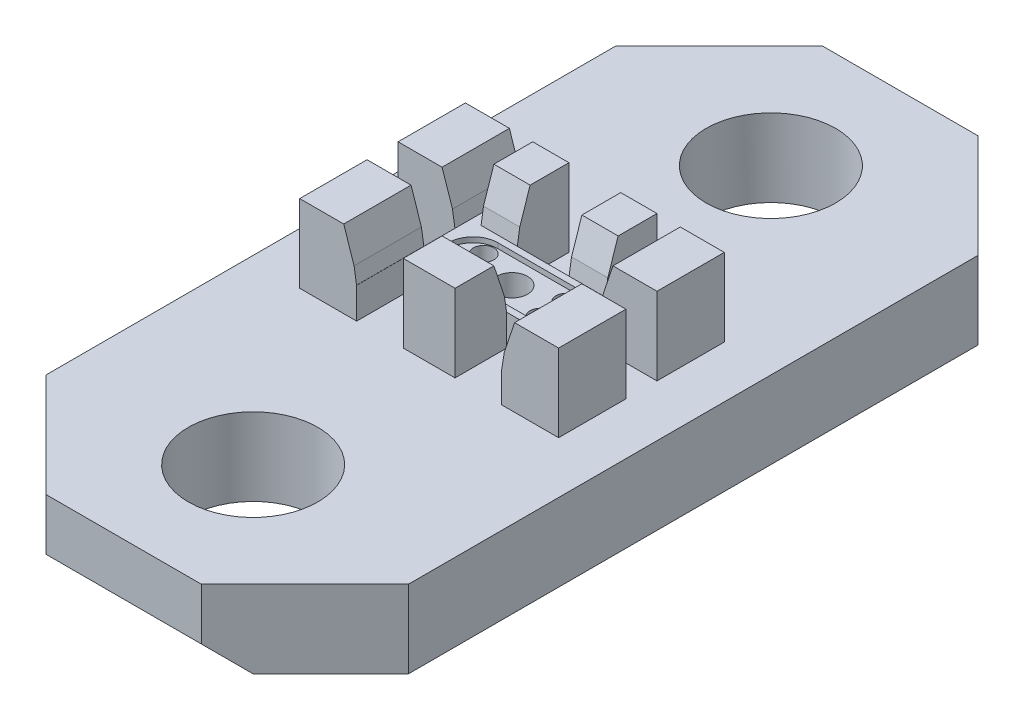
from build123d import *
from OCP.BRepFilletAPI import BRepFilletAPI_MakeChamfer

# Parameters (mm, degrees)
SKETCH1_W           = 7
SKETCH1_H           = 15
BOSS_EXTRUDE1_DEPTH = 1.5
SKETCH2_W           = 5
SKETCH2_H           = 3.2
BOSS_EXTRUDE2_DEPTH = 1.5
SKETCH3_W           = 2.9
SKETCH3_H           = 1.3
CUT_EXTRUDE1_DEPTH  = 0.9
CUT_EXTRUDE2_DEPTH  = 1
CHAMFER1_SIZE       = 0.2
CHAMFER1_SIZE2      = 0.6
CHAMFER2_SIZE       = 0.2
CHAMFER2_SIZE2      = 0.6
CHAMFER3_SIZE       = 2
SKETCH8_R           = 1.25
CUT_EXTRUDE6_DEPTH  = 2
SKETCH9_R           = 0.2
CUT_EXTRUDE7_DEPTH  = 9.538735269
CUT_EXTRUDE8_DEPTH  = 0.1
BOSS_EXTRUDE3_DEPTH = 1.55
BOSS_EXTRUDE4_DEPTH = 0.65
CUT_EXTRUDE3_REACH  = 10.803
SKETCH5_W           = 1
SKETCH5_H           = 5.897515332
CUT_EXTRUDE4_REACH  = 10.803
SKETCH6_W           = 1.097515332
SKETCH6_H           = 0.6
CUT_EXTRUDE5_REACH  = 10.803
SKETCH7_W           = 0.9
SKETCH7_H           = 0.997515332
CHAMFER5_SIZE       = 0.25
CHAMFER5_SIZE2      = 0.6
CUT_EXTRUDE9_DEPTH  = 1.3
CUT_EXTRUDE10_DEPTH = 3.3
SKETCH19_R          = 0.3
CUT_EXTRUDE11_DEPTH = 10
CHAMFER6_SIZE       = 0.5


with BuildPart() as part:
    # Sketch1 → Boss-Extrude1 (new body)
    with BuildSketch(Plane(origin=(0, 0, 0), x_dir=(1, 0, 0), z_dir=(0, 1, 0))):
        Rectangle(SKETCH1_W, SKETCH1_H)
    extrude(amount=BOSS_EXTRUDE1_DEPTH)

    # Sketch2 → Boss-Extrude2 (add)
    with BuildSketch(Plane(origin=(0, 1.5, 0), x_dir=(1, 0, 0), z_dir=(0, 1, 0))):
        Rectangle(SKETCH2_W, SKETCH2_H)
    extrude(amount=BOSS_EXTRUDE2_DEPTH)

    # Sketch3 → Cut-Extrude1 (cut)
    with BuildSketch(Plane(origin=(0, 3, 0), x_dir=(1, 0, 0), z_dir=(0, 1, 0))):
        Rectangle(SKETCH3_W, SKETCH3_H)
    extrude(amount=-CUT_EXTRUDE1_DEPTH, mode=Mode.SUBTRACT)

    # Sketch4 → Cut-Extrude2 (cut)
    with BuildSketch(Plane.XZ):
        with BuildLine():
            Line((-0.75, 0.6), (0.75, 0.6))
            ThreePointArc((0.75, 0.6), (1.35, 0), (0.75, -0.6))
            Line((0.75, -0.6), (-0.75, -0.6))
            ThreePointArc((-0.75, -0.6), (-1.35, 0), (-0.75, 0.6))
        make_face()
    extrude(amount=-CUT_EXTRUDE2_DEPTH, mode=Mode.SUBTRACT)

    # Chamfer1
    chamfer1_edges = [part.edges().sort_by_distance(p)[0] for p in [
        (0, 3, -0.65),
        (0, 3, 0.65),
    ]]
    chamfer1_side = [part.faces().sort_by_distance(p)[0] for p in [
        (-2.440636712, 3, 0),
    ]]
    chamfer(chamfer1_edges, length=CHAMFER1_SIZE, length2=CHAMFER1_SIZE2, reference=chamfer1_side[0])

    # Chamfer2
    chamfer2_edges = [part.edges().sort_by_distance(p)[0] for p in [
        (-1.45, 3, 0),
        (1.45, 3, 0),
    ]]
    chamfer2_side = [part.faces().sort_by_distance(p)[0] for p in [
        (0, 3, -0.909363288),
    ]]
    chamfer(chamfer2_edges, length=CHAMFER2_SIZE, length2=CHAMFER2_SIZE2, reference=chamfer2_side[0])

    # Chamfer3
    chamfer3_edges = [part.edges().sort_by_distance(p)[0] for p in [
        (3.5, 0.75, 7.5),
        (-3.5, 0.75, 7.5),
        (-3.5, 0.75, -7.5),
        (3.5, 0.75, -7.5),
    ]]
    chamfer(chamfer3_edges, length=CHAMFER3_SIZE)

    # Sketch8 → Cut-Extrude6 (cut)
    with BuildSketch(Plane(origin=(0, 1.5, 0), x_dir=(1, 0, 0), z_dir=(0, 1, 0))):
        with Locations(Location((0, -5, 0), (0, 0, 270))):
            Circle(SKETCH8_R)
        with Locations(Location((0, 5, 0), (0, 0, 270))):
            Circle(SKETCH8_R)
    extrude(amount=-CUT_EXTRUDE6_DEPTH, mode=Mode.SUBTRACT)

    # Sketch9 → Cut-Extrude7 (cut, through all)
    with BuildSketch(Plane(origin=(0, 2.1, 0), x_dir=(1, 0, 0), z_dir=(0, 1, 0))):
        with Locations(Location((-0.8, 0.25, 0), (0, 0, 270))):
            Circle(SKETCH9_R)
        with Locations(Location((0.8, 0.25, 0), (0, 0, 90))):
            Circle(SKETCH9_R)
        with Locations(Location((0.8, -0.25, 0), (0, 0, 270))):
            Circle(SKETCH9_R)
        with Locations(Location((-0.8, -0.25, 0), (0, 0, 90))):
            Circle(SKETCH9_R)
    extrude(amount=-CUT_EXTRUDE7_DEPTH, mode=Mode.SUBTRACT)

    # Sketch10 → Cut-Extrude8 (cut)
    with BuildSketch(Plane(origin=(0, 2.1, 0), x_dir=(1, 0, 0), z_dir=(0, 1, 0))):
        with BuildLine():
            Line((-0.75, 0.475), (0.75, 0.475))
            ThreePointArc((0.75, 0.475), (1.225, 0), (0.75, -0.475))
            Line((0.75, -0.475), (-0.75, -0.475))
            ThreePointArc((-0.75, -0.475), (-1.225, 0), (-0.75, 0.475))
        make_face()
    extrude(amount=-CUT_EXTRUDE8_DEPTH, mode=Mode.SUBTRACT)

    # Sketch12 → Boss-Extrude3 (add, symmetric)
    with BuildSketch(Plane(origin=(0, 0, 0), x_dir=(0, 0, -1), z_dir=(1, 0, 0))):
        Polygon((-0.65, 2.4), (-0.602484668, 2.1), (-0.65, 2.1), align=None)
        Polygon((0.65, 2.1), (0.65, 2.4), (0.602484668, 2.1), align=None)
    extrude(amount=BOSS_EXTRUDE3_DEPTH, both=True)

    # Sketch15 → Boss-Extrude4 (add, symmetric)
    with BuildSketch(Plane.XY):
        Polygon((-1.45, 2.4), (-1.402484668, 2.1), (-1.45, 2.1), align=None)
        Polygon((1.45, 2.1), (1.45, 2.4), (1.402484668, 2.1), align=None)
    extrude(amount=BOSS_EXTRUDE4_DEPTH, both=True)

    # Cut-Extrude3: up to this face of the body (flat: up to its plane)
    cut_extrude3_end = Plane(part.part.faces().sort_by_distance((0, 1.5, -7.334470546))[0])
    # Sketch5 → Cut-Extrude3 (cut, up to the picked face)
    with BuildSketch(Plane(origin=(0, 3, 0), x_dir=(1, 0, 0), z_dir=(0, 1, 0)), mode=Mode.PRIVATE) as cut_extrude3_sk1:
        with Locations((0, 3.551242334)):
            Rectangle(SKETCH5_W, SKETCH5_H)
    cut_extrude3_tool1 = split(extrude(cut_extrude3_sk1.sketch, amount=-CUT_EXTRUDE3_REACH, mode=Mode.PRIVATE), bisect_by=cut_extrude3_end, keep=Keep.BOTH, mode=Mode.PRIVATE)
    add(cut_extrude3_tool1.solids().sort_by(Axis((0, 3, -3.551242), (0, -1, 0)))[0], mode=Mode.SUBTRACT)

    # Cut-Extrude4: up to this face of the body (flat: up to its plane)
    cut_extrude4_end = Plane(part.part.faces().sort_by_distance((0, 1.5, -7.334470546))[0])
    # Sketch6 → Cut-Extrude4 (cut, up to the picked face)
    with BuildSketch(Plane(origin=(0, 3, 0), x_dir=(1, 0, 0), z_dir=(0, 1, 0)), mode=Mode.PRIVATE) as cut_extrude4_sk1:
        with Locations((-1.951242334, 0)):
            Rectangle(SKETCH6_W, SKETCH6_H)
    cut_extrude4_tool1 = split(extrude(cut_extrude4_sk1.sketch, amount=-CUT_EXTRUDE4_REACH, mode=Mode.PRIVATE), bisect_by=cut_extrude4_end, keep=Keep.BOTH, mode=Mode.PRIVATE)
    # Sketch6 → Cut-Extrude4 (cut, up to the picked face)
    with BuildSketch(Plane(origin=(0, 3, 0), x_dir=(1, 0, 0), z_dir=(0, 1, 0)), mode=Mode.PRIVATE) as cut_extrude4_sk2:
        with Locations((1.951242334, 0)):
            Rectangle(SKETCH6_W, SKETCH6_H)
    cut_extrude4_tool2 = split(extrude(cut_extrude4_sk2.sketch, amount=-CUT_EXTRUDE4_REACH, mode=Mode.PRIVATE), bisect_by=cut_extrude4_end, keep=Keep.BOTH, mode=Mode.PRIVATE)
    add(cut_extrude4_tool1.solids().sort_by(Axis((-1.951242, 3, 0), (0, -1, 0)))[0], mode=Mode.SUBTRACT)
    add(cut_extrude4_tool2.solids().sort_by(Axis((1.951242, 3, 0), (0, -1, 0)))[0], mode=Mode.SUBTRACT)

    # Cut-Extrude5: up to this face of the body (flat: up to its plane)
    cut_extrude5_end = Plane(part.part.faces().sort_by_distance((0, 1.5, -7.334470546))[0])
    # Sketch7 → Cut-Extrude5 (cut, up to the picked face)
    with BuildSketch(Plane(origin=(0, 3, 0), x_dir=(1, 0, 0), z_dir=(0, 1, 0)), mode=Mode.PRIVATE) as cut_extrude5_sk1:
        with Locations((-0.95, -1.101242334)):
            Rectangle(SKETCH7_W, SKETCH7_H)
    cut_extrude5_tool1 = split(extrude(cut_extrude5_sk1.sketch, amount=-CUT_EXTRUDE5_REACH, mode=Mode.PRIVATE), bisect_by=cut_extrude5_end, keep=Keep.BOTH, mode=Mode.PRIVATE)
    # Sketch7 → Cut-Extrude5 (cut, up to the picked face)
    with BuildSketch(Plane(origin=(0, 3, 0), x_dir=(1, 0, 0), z_dir=(0, 1, 0)), mode=Mode.PRIVATE) as cut_extrude5_sk2:
        with Locations((0.95, -1.101242334)):
            Rectangle(SKETCH7_W, SKETCH7_H)
    cut_extrude5_tool2 = split(extrude(cut_extrude5_sk2.sketch, amount=-CUT_EXTRUDE5_REACH, mode=Mode.PRIVATE), bisect_by=cut_extrude5_end, keep=Keep.BOTH, mode=Mode.PRIVATE)
    add(cut_extrude5_tool1.solids().sort_by(Axis((-0.95, 3, 1.101242), (0, -1, 0)))[0], mode=Mode.SUBTRACT)
    add(cut_extrude5_tool2.solids().sort_by(Axis((0.95, 3, 1.101242), (0, -1, 0)))[0], mode=Mode.SUBTRACT)

    # Chamfer5: one chamfer whose edges measure the first distance from different faces: ONE call of the kernel's chamfer builder (chamfer() names one face for all edges)
    chamfer5_edges_1 = [part.edges().sort_by_distance(p)[0] for p in [
        (1.4, 3, 1.225),
    ]]
    chamfer5_side_1 = [part.faces().sort_by_distance(p)[0] for p in [
        (1.995212766, 3, 0.989893617),
    ]]
    chamfer5_edges_2 = [part.edges().sort_by_distance(p)[0] for p in [
        (-1.4, 3, 1.225),
    ]]
    chamfer5_side_2 = [part.faces().sort_by_distance(p)[0] for p in [
        (-1.995212766, 3, 0.989893617),
    ]]
    chamfer5 = BRepFilletAPI_MakeChamfer(part.part.solid().wrapped)
    for e in chamfer5_edges_1:
        chamfer5.Add(CHAMFER5_SIZE, CHAMFER5_SIZE2, e.wrapped, chamfer5_side_1[0].wrapped)  # the first distance lies on this face
    for e in chamfer5_edges_2:
        chamfer5.Add(CHAMFER5_SIZE, CHAMFER5_SIZE2, e.wrapped, chamfer5_side_2[0].wrapped)  # the first distance lies on this face
    add(Compound.cast(chamfer5.Shape()), mode=Mode.REPLACE)

    # Sketch16 → Cut-Extrude9 (cut)
    with BuildSketch(Plane.XY.offset(1.6)):
        Polygon((-1.45, 2.4), (-1.65, 3), (-1.4, 2.4), (-1.320280654, 2.4), (-1.320280654, 2.1), (-1.402484668, 2.1), align=None)
        Polygon((1.320280654, 2.4), (1.320280654, 2.1), (1.402484668, 2.1), (1.45, 2.4), (1.65, 3), (1.4, 2.4), align=None)
    extrude(amount=-CUT_EXTRUDE9_DEPTH, mode=Mode.SUBTRACT)

    # Sketch18 → Cut-Extrude10 (cut)
    with BuildSketch(Plane.XY.offset(1.6)):
        Polygon((-1.402484668, 2.1), (-1.2, 2.1), (-1.2, 3.166690018), (-1.705563339, 3.166690018), (-1.45, 2.4), align=None)
        Polygon((1.45, 2.4), (1.402484668, 2.1), (1.2, 2.1), (1.2, 3.166690018), (1.705563339, 3.166690018), align=None)
    extrude(amount=-CUT_EXTRUDE10_DEPTH, mode=Mode.SUBTRACT)

    # Sketch19 → Cut-Extrude11 (cut)
    with BuildSketch(Plane.XZ.offset(-1)):
        with Locations(Location((0, 0, 0), (0, 0, 270))):
            Circle(SKETCH19_R)
    extrude(amount=-CUT_EXTRUDE11_DEPTH, mode=Mode.SUBTRACT)

    # Chamfer6
    chamfer6_edges = [part.edges().sort_by_distance(p)[0] for p in [
        (0, 0, -7.5),
        (0, 0, 7.5),
        (-3.5, 0, 0),
    ]]
    chamfer(chamfer6_edges, length=CHAMFER6_SIZE)


solid = part.part
